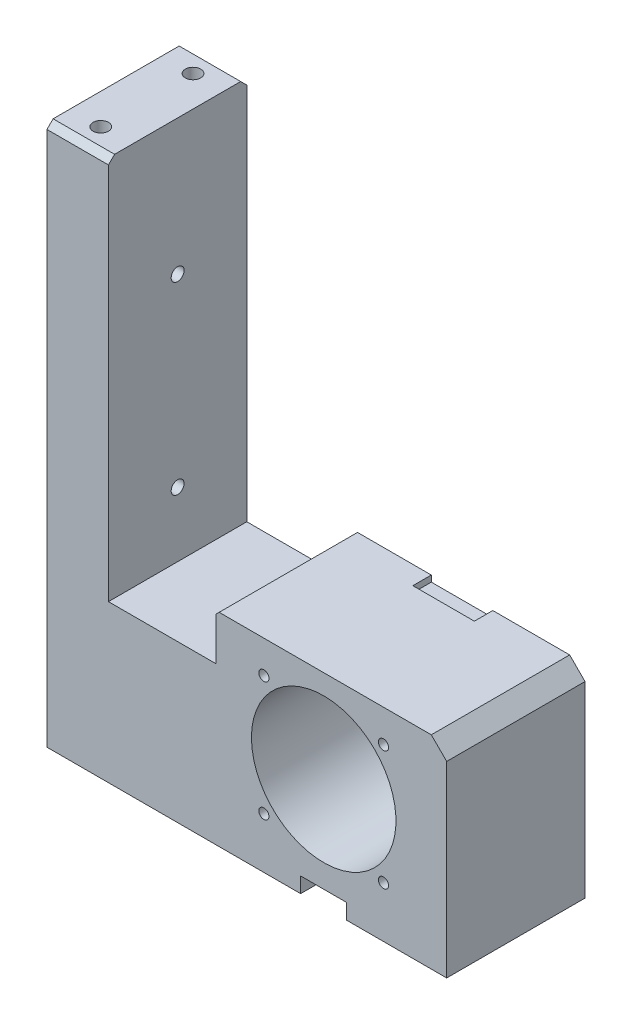
SolidWorks part; units mm, degrees
ref_plane "Front Plane" through (0, 0, 0) normal (0, 0, 1) x (1, 0, 0)
ref_plane "Top Plane" through (0, 0, 0) normal (0, 1, 0) x (1, 0, 0)
ref_plane "Right Plane" through (0, 0, 0) normal (1, 0, 0) x (0, 0, -1)
sketch "Sketch1" plane through (0, 0, 0) normal (0, 0, 1) x (1, 0, 0)
  line L0 (-90, 140) -> (-90, -36)
  line L1 (-90, -36) -> (-7.5, -36)
  line L2 (7.5, -36) -> (40, -36)
  line L4 (40, -36) -> (40, 30)
  line L5 (-70, 140) -> (-70, 30)
  line L6 (-70, 30) -> (40, 30)
  line L7 (-90, 140) -> (-70, 140)
  line L8 (-7.5, -36) -> (-7.5, -31)
  line L9 (-7.5, -31) -> (7.5, -31)
  line L10 (7.5, -36) -> (7.5, -31)
  circle A0 centre (0, 0) radius 23.5
  dimension "D1" = 47
  dimension "D3" = 30
  dimension "D2" = 130
  dimension "D4" = 40
  dimension "D5" = 176
  dimension "D6" = 66
  dimension "D7" = 20
  dimension "D8" = 15
  dimension "D9" = 32.5
  dimension "D10" = 5
extrude "Boss-Extrude1" add sketch "Sketch1" along normal blind 45
hole_wizard "M6 Tapped Hole1" positions "Sketch3" profile "Sketch2" tap size "M6" standard "Gb"
sketch "Sketch3" plane through (0, -36, 0) normal (0, -1, 0) x (1, 0, 0)
  line L0 (-90, 0) -> (-7.5, 0) construction
  line L2 (40, 45) -> (40, 0) construction
  point P0 (-75, 8)
  point P3 (25, 8)
  point P10 (-75, 26)
  point P12 (25, 26)
  dimension "D1" = 8
  dimension "D2" = 100
  dimension "D4" = 15
  dimension "D5" = 18
sketch "Sketch2" plane through (-75, -36, 8) normal (1, 0, 0) x (0, 0, -1)
  line L0 (0, 0) -> (0, 16.5022)
  line L1 (0, 16.5022) -> (2.5, 15)
  line L2 (2.5, 15) -> (2.5, 0)
  line L5 (2.5, 0) -> (0, 0)
  line L10 (0, 16.5022) -> (-2.5, 15) construction
  line L11 (0, -6.35) -> (0, 107.95) construction
  dimension "螺纹孔钻头直径" = 5
  dimension "螺纹孔钻头深度" = 15
  dimension "导头角度" = 118
cosmetic thread "Cosmetic Thread2" parameters "D1"=12, "D2"=6
cosmetic thread "Cosmetic Thread3" parameters "D1"=12, "D2"=6
cosmetic thread "Cosmetic Thread4" parameters "D1"=12, "D2"=6
cosmetic thread "Cosmetic Thread16" parameters "D1"=12, "D2"=6
hole_wizard "M5 Tapped Hole1" positions "Sketch7" profile "Sketch6" tap size "M5" standard "GB" end condition through all
sketch "Sketch7" plane through (-70, 0, 0) normal (1, 0, 0) x (0, 0, -1)
  line L0 (-45, 140) -> (0, 140) construction
  line L1 (-45, 30) -> (-45, 140) construction
  point P0 (-22.5, 96)
  point P1 (-22.5, 36)
  dimension "D1" = 60
  dimension "D2" = 44
  dimension "D3" = 22.5
cosmetic thread "Cosmetic Thread8" parameters "D2"=5
sketch "Sketch6" plane through (-70, 96, 22.5) normal (0, 1, 0) x (0, 0, -1)
  line L0 (0, 0) -> (0, 20)
  line L1 (0, 20) -> (2.1, 20)
  line L2 (2.1, 20) -> (2.1, 0)
  line L5 (2.1, 0) -> (0, 0)
  line L11 (0, -6.35) -> (0, 107.95) construction
  dimension "通孔螺纹孔钻头直径" = 4.2
  dimension "通孔螺纹孔钻头深度" = 20
cosmetic thread "Cosmetic Thread23" parameters "D2"=5
hole_wizard "M6 Tapped Hole2" positions "Sketch9" profile "Sketch8" tap size "M6" standard "GB"
sketch "Sketch9" plane through (0, 140, 0) normal (0, 1, 0) x (-1, 0, 0)
  line L1 (90, 45) -> (90, 0) construction
  line L2 (70, 0) -> (90, 0) construction
  point P0 (80, 7.5)
  point P1 (80, 37.5)
  dimension "D1" = 30
  dimension "D2" = 7.5
  dimension "D3" = 10
sketch "Sketch8" plane through (-80, 140, 7.5) normal (1, 0, 0) x (0, 0, 1)
  line L0 (0, 0) -> (0, 16.5022)
  line L1 (0, 16.5022) -> (2.5, 15)
  line L2 (2.5, 15) -> (2.5, 0)
  line L5 (2.5, 0) -> (0, 0)
  line L10 (0, 16.5022) -> (-2.5, 15) construction
  line L11 (0, -6.35) -> (0, 107.95) construction
  dimension "螺纹孔钻头直径" = 5
  dimension "螺纹孔钻头深度" = 15
  dimension "导头角度" = 118
cosmetic thread "Cosmetic Thread9" parameters "D1"=12, "D2"=6
cosmetic thread "Cosmetic Thread10" parameters "D1"=12, "D2"=6
hole_wizard "M4 Tapped Hole1" positions "Sketch12" profile "Sketch11" tap size "M4" standard "GB"
sketch "Sketch12" plane through (0, 0, 45) normal (0, 0, 1) x (1, 0, 0)
  line L0 (-19.4454, 19.4454) -> (19.4454, -19.4454) construction
  line L1 (-19.4454, -19.4454) -> (19.4454, 19.4454) construction
  line L2 (0, 27.5) -> (0, -27.5) construction
  circle A0 centre (0, 0) radius 27.5 construction
  point P30 (-19.4454, -19.4454)
  point P32 (19.4454, -19.4454)
  point P34 (19.4454, 19.4454)
  point P36 (-19.4454, 19.4454)
  dimension "D1" = 55
  dimension "D2" = 45
  dimension "D3" = 45
sketch "Sketch11" plane through (-19.4454, -19.4454, 45) normal (1, 0, 0) x (0, -1, 0)
  line L0 (0, 0) -> (0, 11.0914)
  line L1 (0, 11.0914) -> (1.65, 10.1)
  line L2 (1.65, 10.1) -> (1.65, 0)
  line L5 (1.65, 0) -> (0, 0)
  line L10 (0, 11.0914) -> (-1.65, 10.1) construction
  line L11 (0, -6.35) -> (0, 107.95) construction
  dimension "螺纹孔钻头直径" = 3.3
  dimension "螺纹孔钻头深度" = 10.1
  dimension "导头角度" = 118
cosmetic thread "Cosmetic Thread11" parameters "D1"=8, "D2"=4
cosmetic thread "Cosmetic Thread12" parameters "D1"=8, "D2"=4
cosmetic thread "Cosmetic Thread13" parameters "D1"=8, "D2"=4
cosmetic thread "Cosmetic Thread14" parameters "D1"=8, "D2"=4
chamfer "Chamfer1" distance 5 angle 45 1 edges at (40, 30, 22.5)
chamfer "Chamfer2" distance 2 angle 45 2 edges at (-80, 140, 0) (-80, 140, 45)
sketch "Sketch15" plane through (0, 0, 45) normal (0, 0, 1) x (1, 0, 0)
  line L1 (-70, 30) -> (-35, 30)
  line L2 (-70, 30) -> (-70, 15)
  line L3 (-70, 15) -> (-35, 15)
  line L4 (-35, 30) -> (-35, 15)
  dimension "D1" = 35
  dimension "D2" = 15
extrude "Cut-Extrude1" cut sketch "Sketch15" against normal through all
chamfer "Chamfer3" distance 1 angle 45 1 edges at (-35, 30, 22.5)
sketch "Sketch18" plane through (0, 30, 0) normal (0, 1, 0) x (1, 0, 0)
  line L0 (35, 0) -> (-34, 0) construction
  line L1 (-10, 0) -> (10, 0)
  line L2 (-10, 0) -> (-10, -6)
  line L3 (-10, -6) -> (10, -6)
  line L4 (10, 0) -> (10, -6)
  line L5 (0, 0) -> (0, -20.0364) construction
  dimension "D1" = 20
  dimension "D2" = 6
extrude "Cut-Extrude2" cut sketch "Sketch18" against normal blind 2
